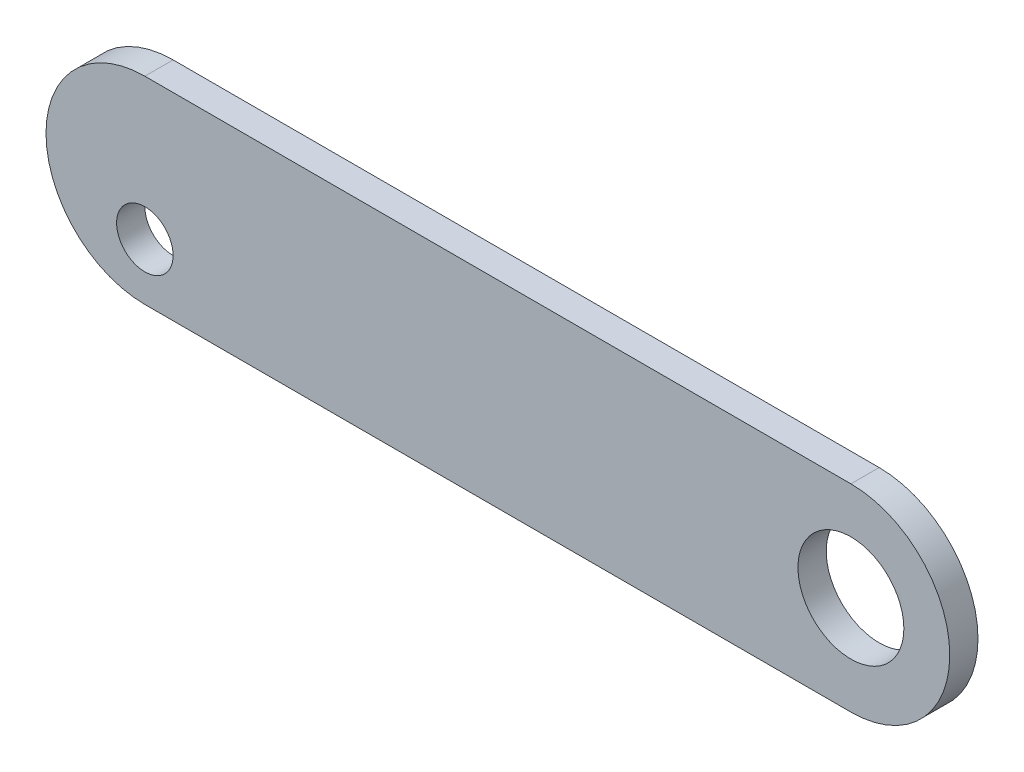
SolidWorks part; units mm, degrees
ref_plane "前视基准面" through (0, 0, 0) normal (0, 0, 1) x (1, 0, 0)
ref_plane "上视基准面" through (0, 0, 0) normal (0, 1, 0) x (1, 0, 0)
ref_plane "右视基准面" through (0, 0, 0) normal (1, 0, 0) x (0, 0, -1)
other "Configuration Table"
sketch "草图1" plane through (0, 0, 0) normal (0, 0, 1) x (1, 0, 0)
  line L0 (-250, 0) -> (250, 0) construction
  line L1 (-250, 70) -> (250, 70)
  line L2 (-250, -70) -> (250, -70)
  arc A0 (-250, 70) -> (-250, -70) centre (-250, 0) ccw
  arc A1 (250, -70) -> (250, 70) centre (250, 0) ccw
  circle A2 centre (250, 0) radius 37.5
  circle A3 centre (-250, -30) radius 20
  point P2 (0, 0)
  dimension "D1" = 75
  dimension "D2" = 70
  dimension "D6" = 40
  dimension "D3" = 250
  dimension "D4" = 40
  dimension "D5" = 250
extrude "凸台-拉伸1" add sketch "草图1" along normal blind 20
